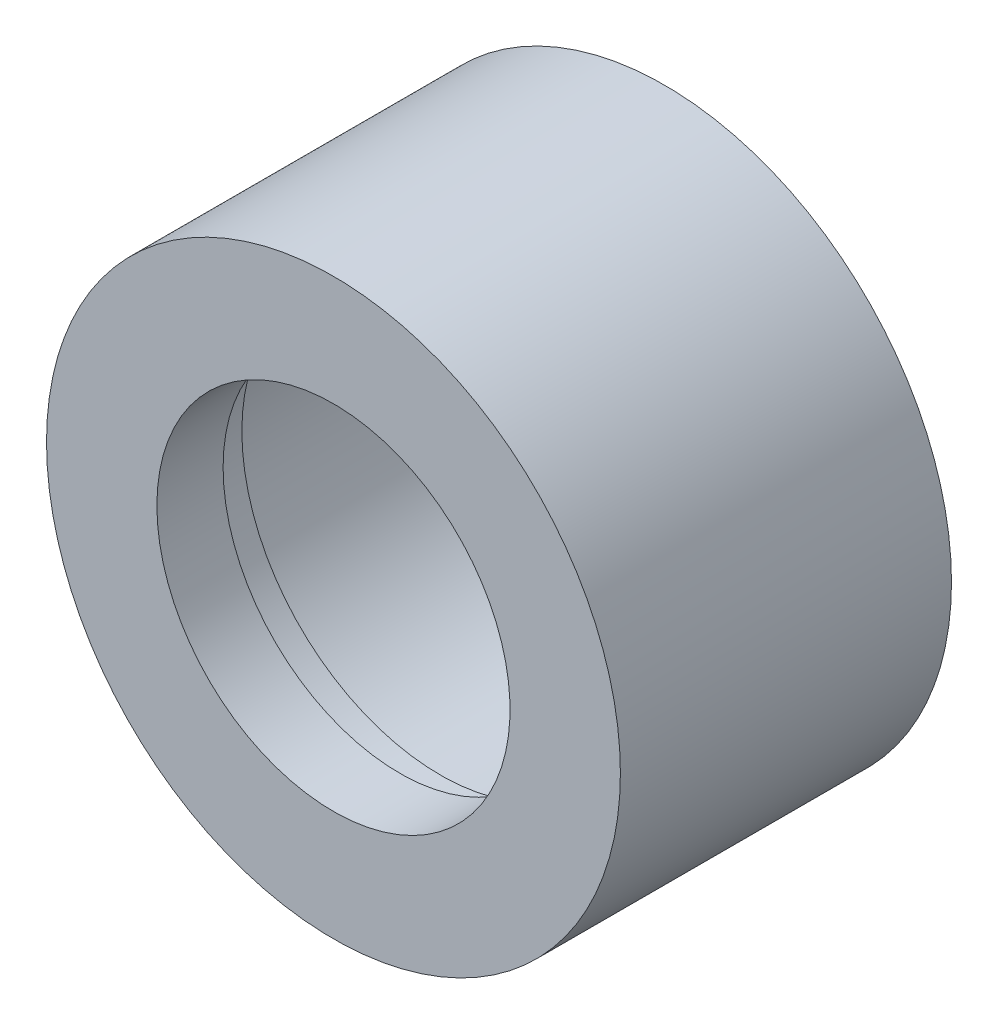
from build123d import *


with BuildPart() as part:
    # Sketch1 → Revolve1 (revolve)
    with BuildSketch(Plane.XZ, mode=Mode.PRIVATE) as revolve1_sk:
        Polygon((9.25, 0), (13, 0), (13, 15), (8, 15), (8, 12), (9, 12), (9, 10.150215155), (9.25, 10), align=None)
    revolve(revolve1_sk.sketch.rotate(Axis((0, 0, 15), (0, 0, -1)), 180), axis=Axis((0, 0, 15), (0, 0, -1)))


solid = part.part
